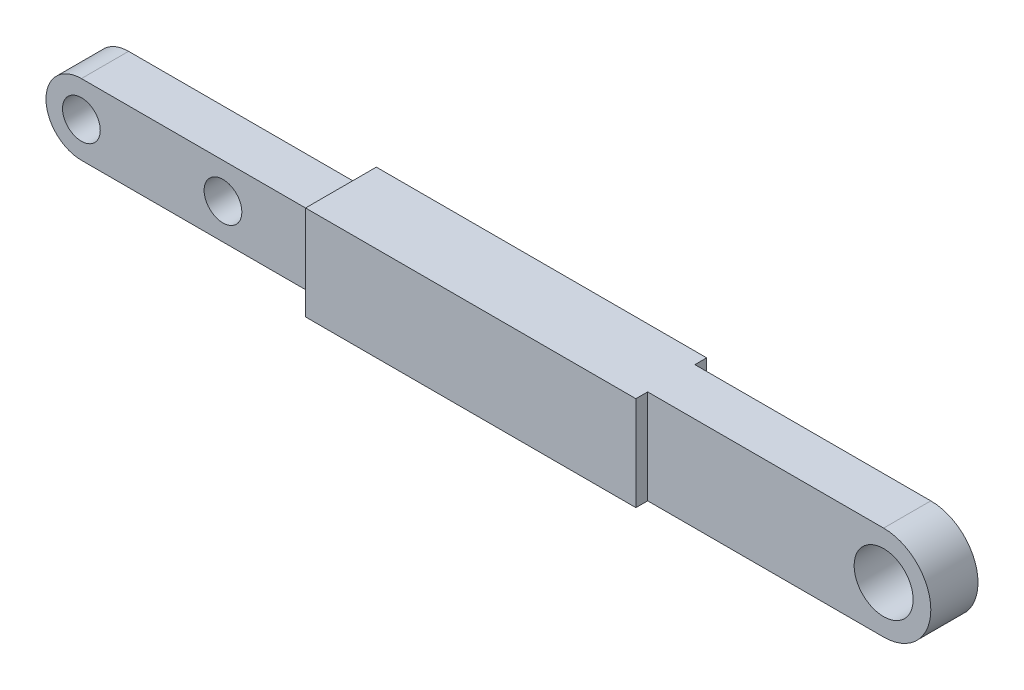
SolidWorks part; units mm, degrees
ref_plane "Front Plane" through (0, 0, 0) normal (0, 0, 1) x (1, 0, 0)
ref_plane "Top Plane" through (0, 0, 0) normal (0, 1, 0) x (1, 0, 0)
ref_plane "Right Plane" through (0, 0, 0) normal (1, 0, 0) x (0, 0, -1)
sketch "Sketch1" plane through (0, 0, 0) normal (0, 0, 1) x (1, 0, 0)
  line L0 (0, -1) -> (0, 1)
  line L1 (0, 1) -> (12, 1)
  line L2 (12, -1) -> (0, -1)
  arc A0 (12, 1) -> (12, -1) centre (12, 0) cw
  circle A1 centre (12, 0) radius 0.625
  dimension "D1" = 1
  dimension "D3" = 1.25
  dimension "D2" = 12
extrude "Boss-Extrude1" add sketch "Sketch1" along normal mid plane 1.5
sketch "Sketch3" plane through (0, 0, 0) normal (0, 0, 1) x (1, 0, 0)
  line L1 (0, 1) -> (0, -1) construction
  line L2 (0, -0.75) -> (-5, -0.75)
  line L3 (-1003.1384, 0) -> (-1.6, 0) construction
  line L4 (0, 0.75) -> (-5, 0.75)
  line L6 (0, 0) -> (1002.1271, 0) construction
  line L7 (0, 0.75) -> (0, -0.75)
  arc A0 (-5, -0.75) -> (-5, 0.75) centre (-5, 0) cw
  circle A1 centre (-5, 0) radius 0.4
  circle A2 centre (-2, 0) radius 0.4
  dimension "D2" = 0.75
  dimension "D3" = 0.8
  dimension "D4" = 3
  dimension "D1" = 5
extrude "Boss-Extrude3" add sketch "Sketch3" along normal mid plane 1
sketch "Sketch6" plane through (0, 0, -0.75) normal (0, 0, -1) x (-1, 0, 0)
  line L0 (-7, 1) -> (-7, -1)
  line L1 (-12, 1) -> (0, 1) construction
  line L2 (0, -1) -> (-12, -1) construction
  line L3 (-7, -1) -> (-12, -1)
  line L4 (-12, 1) -> (-7, 1)
  arc A0 (-12, -1) -> (-12, 1) centre (-12, 0) cw
  dimension "D1" = 5
extrude "Cut-Extrude1" cut sketch "Sketch6" against normal blind 0.25
mirror "Mirror1" about plane through (0, 0, 0) normal (0, 0, 1) of "Cut-Extrude1"
